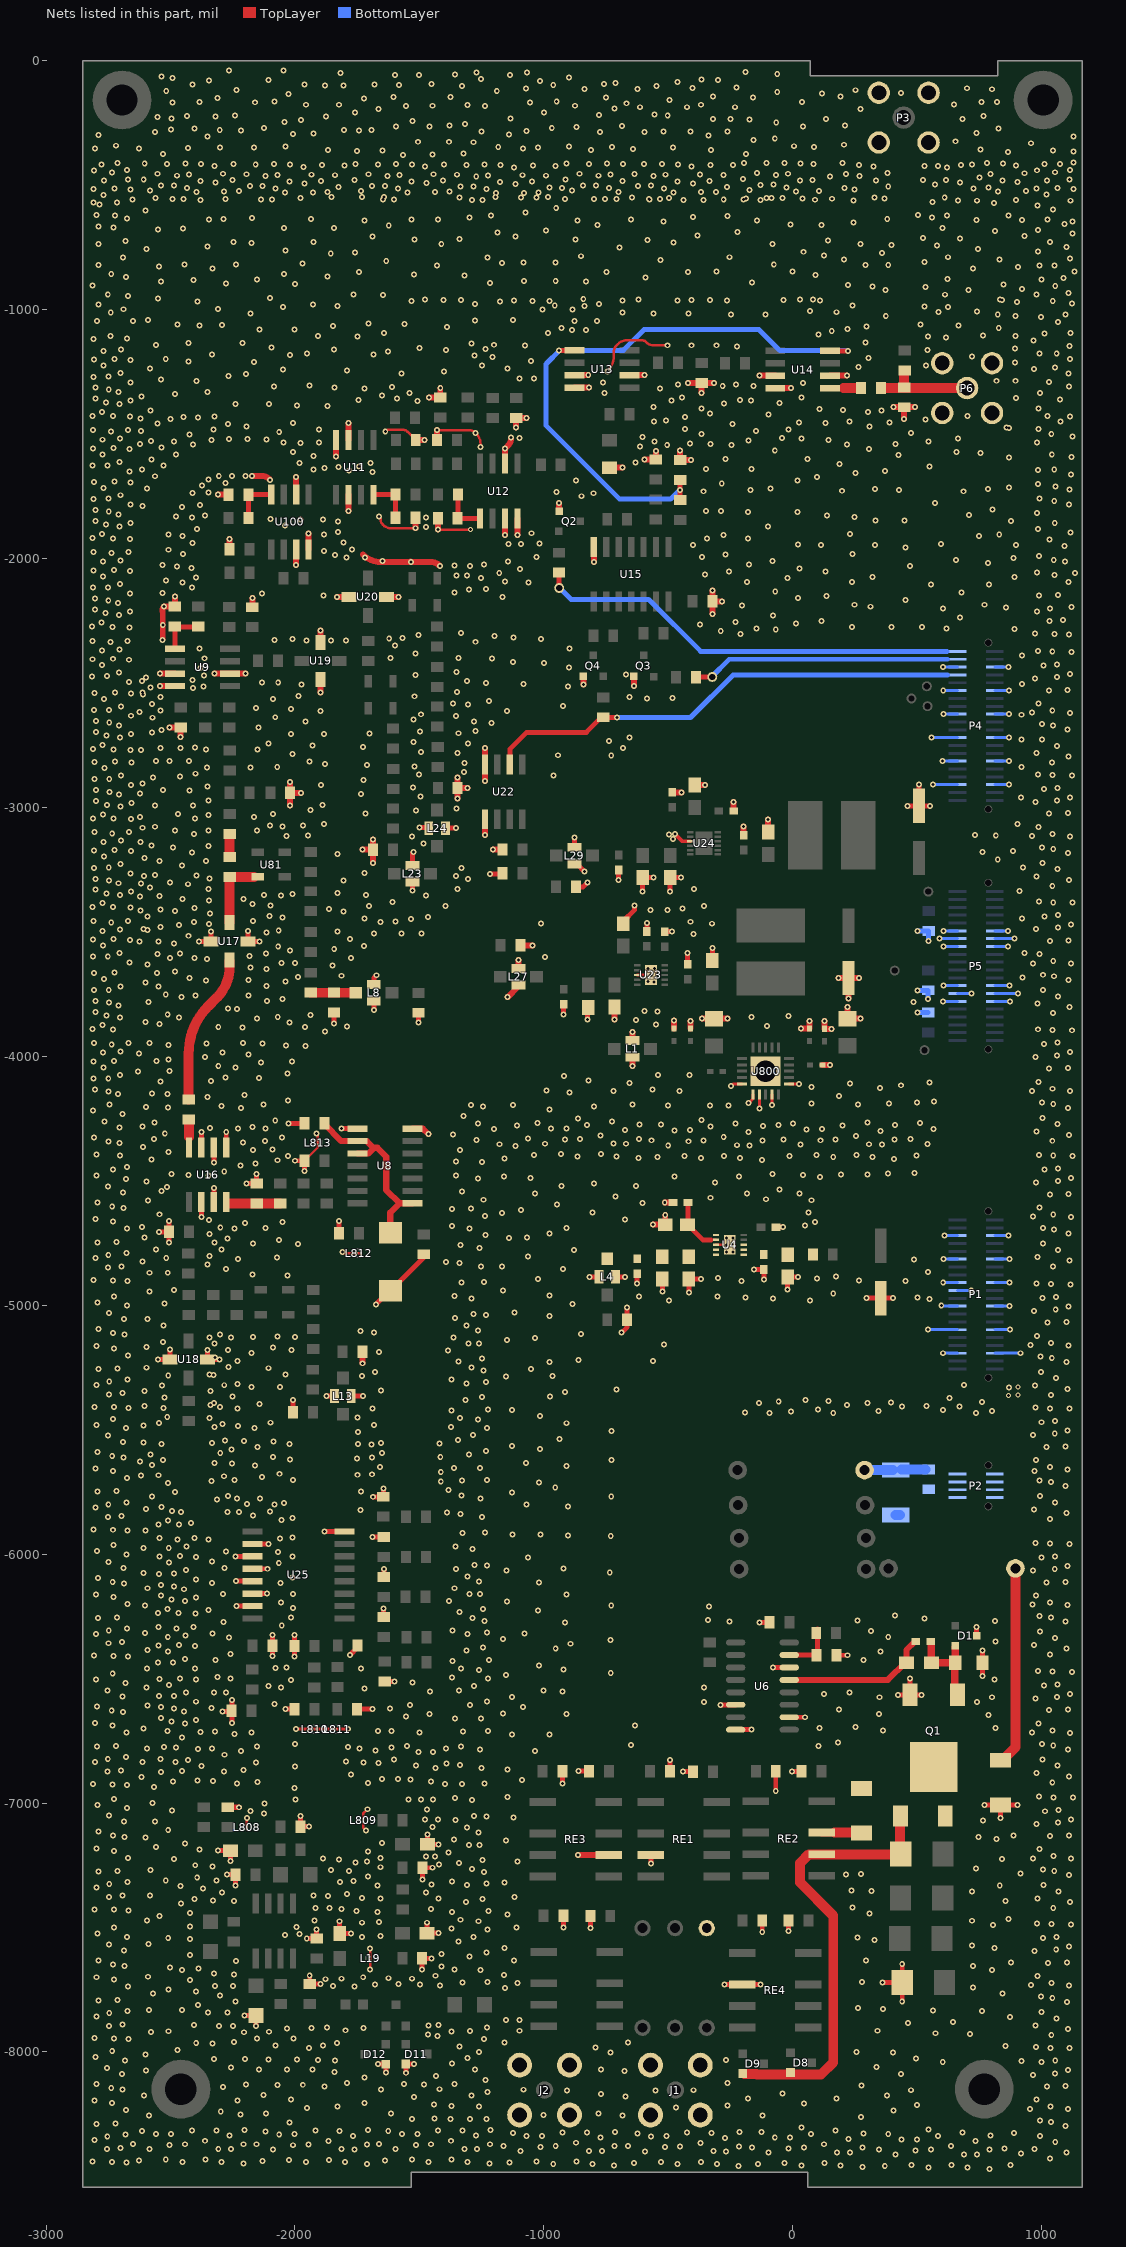
[diagram p0: the nets of this part, all layers, seen from the top]
# Altium PCB MISC109560.PcbDoc (part 5 of 7)
Units mil, origin at the board's own origin, x right, y up, seen from the top; angles counter-clockwise.
Board outline 4015.75 x 8543.31 mil, 4 copper layers (TopLayer, GND, SIG3, BottomLayer); 280 components, 173 nets, 936 pads, 3695 vias.

## Via types
v1: diameter 24, hole 12, TopLayer to BottomLayer, 3659 vias
v2: diameter 20, hole 12, TopLayer to BottomLayer, 32 vias
v3: diameter 40, hole 20, TopLayer to BottomLayer, 4 vias

## Nets (pads, with @x,y where several pads share a name; then routed paths per layer and width w, separated by ;. In a path a pad name is that pad's centre, name@x,y a point inside that pad or via, vN(x,y) a via of type N, cw(c..) or ccw(c..) an arc to the next point about the centre after c; other vN are vias at no path point) (continued)
GND: (continued)
  other v1: -2402,-3044.31 -2811,-3043.31 -2164,-3038.31 -2622,-3037.31 -2348,-3029.31 -2772,-3027.31 -2469,-3026.31 -2088,-3026.31 -1717,-3024.31 1030,-3025 1106,-3023 -1514,-3011.31 -1938,-3009.31 -1351,-3003.61 -2701,-2996.31 -2562,-2992.31 -2409,-2992.31 -1890,-2990.31 -2756,-2989.31 -2657,-2982.31 975,-2978 -2799,-2974.31 -2348,-2972.31 1063,-2972 918,-2960.31 1115,-2959 -1496,-2956.31 -2706,-2948.31 -1735,-2945.31 -2622,-2944.31 -2745,-2937.31 -2424,-2932.31 -2799,-2930.31 -2530,-2929.31 1009,-2926 -1526,-2920.31 1064,-2921 -2351,-2916.31 -1895,-2910.31 -2658,-2909.31 -2613,-2903.31 -1724,-2890.31 -2806,-2886.31 -2746,-2885.31 -2570,-2880.31 -2462,-2875.31 -2698,-2871.31 -961,-2872 1122,-2871 1044,-2870 -1501,-2868.31 986,-2867 -2399,-2864.31 -1321,-2856.61 -2766,-2841.31 -2353,-2839.31 -2179,-2838.31 -2071,-2836.31 919,-2836.31 -1520,-2834.31 -1710,-2829.31 -1879,-2824.31 -1318,-2821 -2657,-2819.31 1042,-2819 -2805,-2817.31 -2722,-2815.31 -1941,-2814.31 -2559,-2812.31 -2504,-2812.31 -2425,-2812.31 1109,-2795 -729,-2791.31 -942,-2790 -2010,-2785.31 -1347,-2780.61 979,-2781 -1493,-2777.31 -2660,-2768.31 -2618,-2768.31 -2357,-2767.31 -2150,-2767.31 -2729,-2766.31 -2812,-2765.31 -681,-2761.31 -2541,-2760.31 -2459,-2760.31 -2402,-2758.31 -1726,-2757.31 1063,-2752 -1929,-2750.31 -2773,-2749.31 -1305,-2743.61 -2107,-2742.31 -1523,-2737.31 -738,-2733.31 919,-2726.31 1002,-2727 -656,-2719.31 -2702,-2718.31 -2757,-2711.31 -2658,-2704.31 -2015,-2704.31 -1883,-2704.31 -1700,-2703.31 -1342,-2701.61 -2575,-2699.31 -2800,-2696.31 -1498,-2695.31 -1274,-2693 -2536,-2689.31 1105,-2687 -2146,-2678.31 -2707,-2670.31 1046,-2671 1001,-2665 -1211,-2661.31 -2746,-2659.31 -1957,-2654.31 -1281,-2654 -2800,-2652.31 -1524,-2647.31 -2572,-2639.31 -2079,-2637.31 -1353,-2633 -2659,-2631.31 919,-2627.31 -1493,-2625.31 1114,-2620 961,-2619 -2624,-2616.31 -1148,-2612.31 -1897,-2611.31 -2541,-2609.31 1043,-2610 -2807,-2608.31 -2747,-2607.31 -2015,-2604.31 -2157,-2600.31 -2699,-2593.31 -923,-2591.31 -1305,-2586.61 -2575,-2583.31 -1365,-2581.61 987,-2582 -1221,-2572.31 -2089,-2564.31 -2767,-2563.31 -585,-2561.31 -483,-2559.31 -2541,-2556.31 -656,-2556.31 -1986,-2552.31 -1519,-2553 -2610,-2546.31 -2658,-2541.31 -2806,-2539.31 -2613,-2538.31 -2723,-2537.31 -1348,-2535.61 1029,-2529 1105,-2527 -2409,-2520.31 -2580,-2517.31 -2368,-2514.31 -903,-2513.31 -1974,-2506.31 922,-2504.31 -1081,-2504 -1233,-2500 -2133,-2497.31 -2067,-2497.31 -2667,-2496.31 -2614,-2491.31 -1308,-2491.61 -2411,-2488.31 974,-2482 -2599,-2477.31 1062,-2476 -2815,-2473.31 -2755,-2472.31 -2366,-2470.31 -1515,-2467 -670,-2465.31 1114,-2463 -2707,-2458.31 -1350,-2455.61 -2379,-2440.31 -899,-2437.31 1008,-2430 -2775,-2428.31 1063,-2425 -1000,-2419 -1123,-2415 -2666,-2406.31 -2814,-2404.31 -2731,-2402.31 -2363,-2400.31 -1208,-2401 -1616,-2399.31 -1342,-2399.61 922,-2389.31 -1515,-2382 1121,-2375 1043,-2374 985,-2371 -2776,-2369.31 -2705,-2364.31 -2384,-2360.31 -897,-2360.31 -1598,-2349.31 -2741,-2335.31 -1274,-2334 -2813,-2330.31 -2673,-2330.31 -1954,-2329.31 -1855,-2329.31 -1794,-2329.31 -2082,-2327.31 -2533,-2326.31 -2009,-2322.31 -1012,-2323 -1621,-2321.31 -1567,-2318 -1122,-2317 -1198,-2311 -1504,-2307 1110,-2305 -210,-2303.31 1052,-2302 974,-2301 -1333,-2299 -289,-2290.31 -68,-2285.31 892,-2283.31 -146,-2280.31 618,-2280.31 -2664,-2276.31 238,-2275.31 398,-2275.31 520,-2275.31 -2733,-2274.31 -2816,-2273.31 -2531,-2266.31 -372,-2264.31 13,-2261.31 -2777,-2257.31 -230,-2254.31 116,-2250.31 1032,-2251 1087,-2246 672,-2237.31 -79,-2229.31 -2706,-2226.31 -2761,-2219.31 -2662,-2212.31 981,-2213 -2804,-2204.31 604,-2201.31 1033,-2200 857,-2196.31 312,-2193.31 1121,-2194 -203,-2188.31 249,-2185.31 770,-2185.31 -2711,-2178.31 -2750,-2167.31 453,-2166.31 -2804,-2160.31 21,-2157.31 -1165,-2154 135,-2150.31 990,-2149 -1885,-2147.31 1066,-2147 -2132,-2140.31 -2663,-2139.31 -2533,-2138.31 678,-2136.31 -1358,-2135.31 -70,-2131.31 -1301,-2124.31 -1232,-2122.31 -2811,-2116.31 -2751,-2115.31 -2414,-2115.31 556,-2104.31 789,-2104.31 -2703,-2101.31 -1062,-2096.31 -2451,-2095.31 -184,-2093.31 238,-2093.31 1108,-2094 -1156,-2092 -2518,-2087.31 -21,-2078.31 -1252,-2077.31 -2397,-2076.31 320,-2074.31 892,-2074.31 -2771,-2071.31 -1350,-2068.31 -1309,-2067.31 1052,-2066 -352,-2063.31 -1179,-2058 1134,-2057 981,-2056 -255,-2052.31 132,-2052.31 -2662,-2049.31 -2810,-2047.31 -2727,-2045.31 -1095,-2042 27,-2040.31 -2415,-2038.31 -2474,-2031.31 472,-2030.31 -1418,-2029.31 -1296,-2029.31 -1358,-2028.31 -2533,-2025.31 -175,-2024.31 -1241,-2023.31 784,-2017.31 -2772,-2012.31 -1649,-2010.31 -1143,-2011 1094,-2011 -82,-2009.31 -2701,-2007.31 656,-2006.31 1049,-2005 887,-1998.31 -1792,-1996.31 -1718,-1995.31 -1029,-1993.31 -364,-1993.31 990,-1989 -1838,-1985.31 -270,-1983.31 241,-1982.31 -2450,-1981.31 -2737,-1978.31 -2809,-1973.31 -2669,-1973.31 -1884,-1969.31 -2507,-1964.31 -1770,-1963.31 453,-1955.31 1093,-1949 -401,-1944.31 114,-1944.31 331,-1944.31 897,-1944.31 21,-1942.31 -1141,-1941.31 -1092,-1941.31 596,-1941.31 -1018,-1939.31 -2411,-1937.31 -1804,-1934.31 1032,-1924 -2662,-1920.31 -2731,-1918.31 -345,-1918.31 -179,-1918.31 -2814,-1917.31 -2452,-1908.31 748,-1908.31 -278,-1904.31 830,-1903.31 -2508,-1902.31 -1883,-1902.31 -2775,-1901.31 230,-1900.31 -1050,-1898 1116,-1895 -1827,-1893.31 -2394,-1881.31 986,-1881 -1473,-1872.31 -2704,-1870.31 -99,-1870.31 -2040,-1866.31 -2759,-1863.31 -2660,-1856.31 1053,-1857 -1826,-1851.31 878,-1849.31 -2802,-1848.31 333,-1846.31 450,-1846.31 -1977,-1843.31 -1888,-1842.31 -2098,-1841.31 -2413,-1835.31 -1473,-1835.31 249,-1832.31 -1663,-1831.31 -2478,-1830.31 138,-1827.31 -2362,-1826.31 708,-1824.31 -2709,-1822.31 981,-1817 -179,-1813.31 20,-1813.31 -2748,-1811.31 -349,-1809.31 -288,-1809.31 -2802,-1804.31 803,-1803.31 -2454,-1792.31 -2612,-1788 -2381,-1784.31 -2661,-1783.31 1111,-1783 572,-1776.31 1051,-1769 -2809,-1760.31 -2749,-1759.31 992,-1759 -849,-1749.31 -2701,-1745.31 -800,-1737.31 -2411,-1736.31 -2347,-1734.31 -949,-1733 -358,-1729.31 686,-1729.31 198,-1727.31 428,-1724.31 -169,-1723.31 1113,-1722 331,-1719.31 784,-1719.31 -2595,-1719 -89,-1717.31 -2769,-1715.31 870,-1713.31 1056,-1710 -2374,-1705.31 986,-1701 -285,-1698.31 -2279,-1695.31 -2660,-1693.31 -2808,-1691.31 -2725,-1689.31 20,-1686.31 -871,-1685.31 -2100,-1684.31 -2347,-1682.31 98,-1671.31 -2563,-1669 -2306,-1668.31 -2253,-1667.31 -2199,-1667.31 1119,-1662 252,-1656.31 -1688,-1651.31 -2665,-1649.31 371,-1647.31 -1782,-1645.31 985,-1643 -1926,-1641.31 -2614,-1641 1051,-1641 -348,-1639.31 -165,-1639.31 -1881,-1636.31 -1825,-1631.31 -1742,-1629.31 550,-1629.31 -2813,-1626.31 -2753,-1625.31 -2528,-1625 188,-1620.31 -1697,-1616.31 -1981,-1615.31 -632,-1614.31 -2705,-1611.31 -2576,-1601 -269,-1599.31 59,-1599.31 870,-1594.31 1121,-1591 -1926,-1587.31 425,-1583.31 -2773,-1581.31 -2477,-1581.31 1041,-1582 754,-1575.31 -2007,-1572.31 659,-1572.31 -72,-1565.31 -2664,-1559.31 306,-1559.31 -2812,-1557.31 -2729,-1555.31 -2536,-1554.31 -1255,-1552.31 -614,-1550.31 -504,-1542.68 -246,-1542.68 -2410,-1541.31 219,-1541.68 -330,-1539.31 -2622,-1539 -412,-1538.31 414,-1538.68 -1978,-1536.31 -2046,-1534.31 -1903,-1534.31 981,-1534 -2486,-1529.31 545,-1529.31 -555,-1528.68 -2578,-1528 -177,-1525.31 -2336,-1523.31 144,-1523.68 -2774,-1522.31 -2114,-1521.31 -2264,-1519.31 -2191,-1519.31 -2703,-1517.31 36,-1517.68 664,-1516.68 -1098,-1515.31 -42,-1514.68 -1131,-1513.31 -604,-1510.68 1124,-1510 -2424,-1501.31 -366,-1498.68 1039,-1499 -1275,-1495.31 476,-1494.68 -2063,-1491.31 -2739,-1488.31 -1637,-1488.31 -2618,-1487.31 -147,-1486.68 -2811,-1483.31 -2671,-1483.31 -16,-1481.68 -2327,-1480.31 -1903,-1480.31 -432,-1479.68 988,-1479 870,-1474.31 859,-1472.31 309,-1469.68 -2194,-1468.31 -242,-1459.68 -2269,-1458.31 -2552,-1456.31 132,-1455.68 -2007,-1454.31 389,-1453.68 25,-1452.68 -558,-1448.68 229,-1448.68 1076,-1449 -509,-1445.68 533,-1440.68 -2499,-1439.31 -2620,-1437.31 -2389,-1432 -433,-1430.68 -2662,-1429.31 -2448,-1430 1114,-1429 -2731,-1427.31 -2323,-1428 702,-1427.68 -2814,-1426.31 1024,-1426 -97,-1421.68 -332,-1417.68 -2775,-1410.31 302,-1410.68 356,-1405.68 -2581,-1404 202,-1403.68 108,-1398.68 -366,-1397.68 988,-1397 -559,-1390.68 -1870,-1387 -1992,-1384 -2704,-1379.31 -2239,-1378 -2105,-1378 -276,-1376.68 -52,-1374.68 -2759,-1372.31 -2660,-1365.31 -1508,-1366 -486,-1364.68 -168,-1364.68 -1744,-1363.31 -211,-1361.68 1074,-1361 -2802,-1357.31 -1590,-1357 897,-1355.31 -445,-1352.68 36,-1352.68 -2616,-1349.31 -1650,-1344.31 -2482,-1339 994,-1335 -1540,-1334 -756,-1333.68 -2709,-1331.31 -2351,-1331 -2748,-1320.31 -1721,-1316.31 -533,-1316.68 -2802,-1313.31 -1841,-1313 -1609,-1311.31 1111,-1309 -2084,-1308 -281,-1305.68 -157,-1305.68 -1941,-1305 -460,-1300.68 -228,-1299.68 41,-1293.68 -2661,-1292.31 -763,-1291.68 1029,-1290 -2396,-1287 819,-1285.31 895,-1285.31 -2538,-1280 -1097,-1277 -1039,-1277 -2809,-1269.31 -2749,-1268.31 -2266,-1267 -2197,-1259 1109,-1257 -1572,-1256 -2701,-1254.31 -1401,-1248 -744,-1247.68 -1790,-1244 -2047,-1240 969,-1238 -2583,-1237 -1145,-1236 1054,-1232 265,-1230.68 -2769,-1224.31 -1248,-1224.31 535,-1223.68 894,-1211.31 -2164,-1209 -2428,-1208 -1052,-1206 -2660,-1202.31 -2808,-1200.31 -2725,-1198.31 1114,-1198 -2519,-1197 304,-1194.68 -1207,-1189.31 721,-1187.68 -1279,-1183.68 -2020,-1182 -2333,-1180 -1684,-1180 -1952,-1176 991,-1175 1061,-1175 -1626,-1167 -2770,-1165.31 541,-1161.68 -2699,-1160.31 -1392,-1161 -1843,-1159 -1234,-1157.31 893,-1156.31 -1499,-1154 -2095,-1151 -224,-1147.68 1112,-1146 -1076,-1144 -406,-1142.68 -306,-1142.68 -2559,-1141 -1201,-1140.68 -1290,-1135.68 -2427,-1133 -2210,-1133 292,-1131 968,-1123 -2810,-1118 -2674,-1115 616,-1110.68 -1748,-1108 543,-1107.68 -2741,-1106 895,-1105.31 -1907,-1105 764,-1103.68 104,-1098.68 1012,-1096 -1642,-1094 1117,-1094 -983,-1092.68 157,-1085 -886,-1081.68 -831,-1081.68 -2002,-1080 -2143,-1079 221,-1077.68 828,-1073.31 -929,-1072.68 -1389,-1069 296,-1068 -1847,-1065 -2384,-1064 666,-1063.68 -2293,-1061 -2472,-1059 514,-1059 -1559,-1057 -1705,-1056 1066,-1050 -2795,-1046 -786,-1046 -2651,-1045 -876,-1045 -1277,-1043 -1124,-1042 -2590,-1041 998,-1030 895,-1025.31 374,-1025 1096,-1020 -247,-1019 -109,-1019 824,-1018.31 -2179,-1015 -559,-1015 -418,-1015 -2740,-1011 -684,-1011 177,-1010 585,-1008.68 741,-1006.31 70,-1005.31 -1005,-998.31 -884,-998.31 -2688,-998 -2310,-997 624,-989.68 -2047,-989 530,-986 -837,-984.31 -1829,-984 -956,-983.31 241,-983 -2790,-979 -1928,-979 -778,-977.31 -1277,-976 1122,-975 902,-968.31 -2392,-967 -1176.43,-966.54 -976.43,-965.54 -1532.43,-964.54 -1045.43,-964.54 -1119.43,-963.54 -463.43,-963.54 1045,-964 -684.43,-962.54 -263.43,-962.54 109,-962.31 -1333.43,-961.54 -332.43,-961.54 -37,-961.31 -1402.43,-960.54 -406.43,-960.54 841.57,-960.54 -1476.43,-959.54 28.57,-959.54 833,-959.31 -620.43,-958.54 81.57,-958.54 -841.43,-957.54 -2551,-954 -2101,-953 -2670,-944 -1646,-941 612,-939.68 -2752,-938 -1764,-938 980,-938 1109,-933 373,-921 706,-920 922,-916 534,-908 321,-907 1055,-905 -2813,-903 223,-900 848,-898 -2000,-897 -2276,-894 -1216,-892 -163,-890 -2538,-887 -831,-887 -1080,-885 -952,-885 -2408,-881 -2153,-879 999,-879 623,-876.68 1089,-872 -592,-871 -2679,-868 -1869,-867 -1319,-863 91,-861 -1522,-859 -2738,-857 -2043,-857 -748,-849 -1742,-848 -420,-848 -307,-846 -1,-846 1133,-846 -2332,-834 724,-834 905,-828 -2546,-826 -1430,-823 992,-823 1052,-823 293,-821 -2790,-820 384,-820 -76,-819 -2443,-818 -2236,-818 -1969,-815 -1167,-813 -1081,-810 -953,-810 530,-809 -1633,-805 -532,-800 206,-799 831,-799 1114,-795 -2691,-790 -1227,-790 -253,-789 625,-789 -850,-785 126,-782 -1856,-774 359,-772 -1759,-770 44,-767 986,-766 -2038,-761 -2597,-756 745,-756 -696,-749 1100,-748 -2351,-746 580,-741 398,-739 -2790,-736 272,-736 -1412,-735 -82,-735 -2174,-731 -478,-729 -1925,-728 1033,-728 -2247,-727 -2680,-723 141,-722 -583,-720 -1520,-718 -873,-718 -1338,-715 672,-714 524,-712 -1113,-706 -1689,-705 932,-704 -383,-702 1125,-693 -1186,-690 -222,-687 813,-683 -992,-681 986,-680 -2551,-677 -2449,-674 -2043,-672 -1843,-672 602,-671 -2729,-669 -2790,-666 -1623,-661 -785,-659 116,-659 -8,-657 1092,-656 244,-650 -519,-646 1125,-645 -1721,-642 -864,-642 -144,-642 739,-640 922,-640 -2346,-638 -1532,-638 -1425,-638 -649,-638 1024,-638 -2287,-636 -1936,-636 380,-636 -2675,-633 -2173,-632 -1299,-630 559,-630 -400,-628 -262,-624 621,-622 -2723,-621 -1212,-621 868,-621 -2797,-620 503,-619 -1074,-609 -2600,-602 1046,-597 -950,-592 984,-581 -2785,-578 808,-572 -2809,-570 -2715,-569 562,-567 741,-562 1116,-562 244,-561 664,-561 -2379,-559.31 -438,-559.31 897.57,-559.54 -1289.43,-558.54 -1245.43,-558.54 -358,-558.31 -128.43,-558.54 -277,-557.31 -197.43,-557.54 90,-558 -2652,-557 -2136.43,-556.54 -2092.43,-556.54 -1645.43,-556.54 -1601.43,-556.54 -576,-556.31 -914,-555.31 -707,-555.31 -576.43,-555.54 -532.43,-555.54 -2492.43,-554.54 -2448.43,-554.54 -2278,-554.31 -797.43,-554.54 -753.43,-554.54 -187,-553.31 39,-553.31 158,-554 369,-553 -2561,-551.31 -105,-551.31 -84.43,-551.54 -40.43,-551.54 -1977,-550.31 -497,-550.31 -1338,-548.31 -1092,-548.31 -1030,-548.31 -645,-548.31 329,-549 611,-549 -1853,-547.31 -1731,-547.31 -1643,-547.31 -983,-547.31 -1194,-546.31 -2769.43,-538.54 1019.57,-537.54 -1192.43,-531.54 -1080.43,-530.54 -2039.43,-529.54 -1548.43,-529.54 -1021.43,-529.54 -1927.43,-528.54 -479.43,-528.54 -2395.43,-527.54 -1868.43,-527.54 -700.43,-527.54 -367.43,-527.54 -1437.43,-526.54 -308.43,-526.54 -1378.43,-525.54 825.57,-525.54 -2284.43,-524.54 12.57,-524.54 -2225.43,-523.54 -1734.43,-523.54 105.57,-523.54 936.57,-522.54 -2581.43,-521.54 -886.43,-521.54 -173.43,-518.54 -2660.43,-516.54 -1230.43,-515.54 248,-516 1128.57,-515.54 -2808.43,-514.54 -2077.43,-513.54 -1586.43,-513.54 980.57,-513.54 -2725.43,-512.54 -517.43,-512.54 -2433.43,-511.54 -738.43,-511.54 726,-512 1063.57,-511.54 -977.43,-509.54 -926,-510 208.12,-509.93 787.57,-509.54 -25.43,-508.54 -1824.43,-507.54 -264.43,-506.54 -1334.43,-505.54 -1282.43,-504.54 384,-505 -2181.43,-503.54 -1690.43,-503.54 -2129.43,-502.54 -1638.43,-502.54 -621.43,-502.54 -2537.43,-501.54 -842.43,-501.54 -569.43,-501.54 -2485.43,-500.54 -790.43,-500.54 -129.43,-498.54 -77.43,-497.54 571,-497 -1114.43,-495.54 -1961.43,-493.54 -401.43,-492.54 -1471.43,-491.54 -2318.43,-489.54 -1175.43,-487.54 673,-488 902.57,-487.54 -2022.43,-485.54 -1531.43,-485.54 -1047.43,-485.54 -462.43,-484.54 -2378.43,-483.54 -1894.43,-483.54 -683.43,-483.54 -334.43,-482.54 -2766.43,-481.54 -1404.43,-481.54 842.57,-481.54 29.57,-480.54 334,-481 1022.57,-480.54 -2251.43,-479.54 -1760.43,-479.54 79.57,-479.54 617,-479 -2607.43,-477.54 -912.43,-477.54 523,-478 1112.57,-477.54 -2671.43,-476.54 -199.43,-474.54 750,-468 -1271.43,-465.54 150.57,-464.23 -2118.43,-463.54 -1627.43,-463.54 -558.43,-462.54 -2474.43,-461.54 -991.43,-461.54 -779.43,-461.54 268,-462 -1223.43,-460.54 -1838.43,-459.54 -1085.43,-459.54 -2070.43,-458.54 -1579.43,-458.54 -278.43,-458.54 -66.43,-458.54 -1932.43,-457.54 -1348.43,-457.54 -510.43,-457.54 -2426.43,-456.54 -731.43,-456.54 -372.43,-456.54 -2195.43,-455.54 -1704.43,-455.54 -1442.43,-455.54 -635.43,-454.54 215.12,-454.93 794.57,-454.54 -2551.43,-453.54 -2289.43,-453.54 -856.43,-453.54 -18.43,-453.54 931.57,-451.54 -143.43,-450.54 381,-450 -2734.43,-448.54 1054.57,-447.54 -2806.43,-440.54 982.57,-439.54 -2675.43,-438.54 1113.57,-437.54 -1119.43,-427.54 621,-428 -1966.43,-425.54 -406.43,-424.54 325,-425 -1476.43,-423.54 -2323.43,-421.54 -953.43,-421.54 530,-422 583,-422 -1043.43,-420.54 -1800.43,-419.54 897.57,-419.54 -1890.43,-418.54 -1173.43,-418.54 -240.43,-418.54 -1310.43,-417.54 -330.43,-417.54 267,-418 676,-418 -2020.43,-416.54 -1529.43,-416.54 -1400.43,-416.54 -1237.43,-416.54 -2776.43,-415.54 -2157.43,-415.54 -1666.43,-415.54 -460.43,-415.54 721,-416 -2376.43,-414.54 -2247.43,-414.54 -2084.43,-414.54 -1756.43,-414.54 -1593.43,-414.54 -681.43,-414.54 -597.43,-414.54 83.57,-414.54 1012.57,-414.54 1074,-415 -2513.43,-413.54 -818.43,-413.54 -524.43,-413.54 -2603.43,-412.54 -2440.43,-412.54 -908.43,-412.54 -745.43,-412.54 844.57,-412.54 31.57,-411.54 -2712.43,-410.54 -105.43,-410.54 201.12,-410.93 780.57,-410.54 -195.43,-409.54 -32.43,-409.54 1128.57,-408.54 -1566.43,-377.54 -1446.43,-376.54 -2529.43,-374.54 -188.43,-373.54 -1323.43,-372.54 866,-366 1128,-364 -1750,-362 -1649,-360 1046,-360 -1868,-358 -810,-358 -328,-358 755,-356 -641,-355 -2804,-353 -2627,-353 -1084,-353 -2429,-351 -2301,-349 -2165,-349 -1023,-349 -480,-349 -1183,-347 -726,-347 85,-347 -2037,-345 -899,-345 6,-343 -2719,-341 206,-337 957,-331 -1282,-327 -1505,-325 -1381,-325 654,-323 -158,-318 -72,-312 -2351,-303.31 1128,-303 -338,-299.31 -2790,-298 -1139,-295.31 -2008,-293.31 -1925,-291.31 738,-290 -774,-286.31 -596,-286.31 -2563,-285 -519,-284.31 -410,-284.31 -262,-284.31 -1250,-283.31 -1069,-282.31 -2217,-279.31 -1742,-279.31 -2302,-278.31 -1692,-278.31 -1803,-277.31 -2497,-275.31 -2404,-271.31 -968,-270.31 827,-271 -2125,-269.31 -868,-265.31 -1594,-264.31 -1460,-264.31 42,-263 -686,-261.31 -1378,-260.31 211,-259 -1316,-253.31 -66,-248 -2042,-246.31 -1527,-241.31 -1975,-237.31 -174,-236.31 -320,-234.31 -249,-233.31 134,-234 683,-234 -2495,-231.31 -1134,-231.31 -2553,-226 -2320,-223.31 -1876,-223.31 -2434,-221.31 767,-222 -502,-220.31 -2241,-219.31 -778,-218.31 -555,-216.31 -1758,-207.31 -1000,-207.31 -1664,-194.31 -715,-192.31 272,-193 -613,-186.31 -425,-186.31 -232,-186.31 -1553,-181.31 -1236,-181.31 -1447,-180.31 -874,-180.31 -1307,-177.31 -1955,-176.31 -1823,-176.31 -368,-176.31 648,-176 -667,-170.31 -2492,-167.31 -1056,-167.31 -2161,-166.31 37,-166 759,-166 821,-166 -2384,-164.31 -2082,-162.31 -948,-162.31 -494,-157.31 -1723,-151.31 -2311,-149.31 -751,-147.31 -159,-146.31 -1604,-145.31 -1375,-145.31 -320,-142.31 192,-143 -2025,-132.31 118,-131 435,-129 -62,-125 -1189,-121.31 -2517,-120.31 252,-118 -2234,-116.31 -837,-113.31 -623,-113.31 800,-114 -1071,-110.31 -402,-109.31 701,-110 -226,-107.31 -1328,-101.31 -548,-101.31 -1880,-99.31 -1805,-99.31 -962,-97.31 -1582,-96.31 -2412,-95.31 -1962,-94.31 -1680,-94.31 -1452,-93.31 -759,-92.31 -711,-88.31 -462,-84.31 -1015,-80.31 -2345,-78.31 -301,-77.31 -2107,-76.31 -366,-74.31 -1252,-73.31 -2492,-69.31 -899,-67.31 -2536,-62.31 -1135,-57.31 -1598,-56 -1501,-56 -1356,-54 -62,-52 -1816,-48 -1270,-46 -1068,-46 -189,-44 -2264,-38 -2045,-38
  other v2: 868,-5362 906,-5360 906,-5329 -265,-4785 -240,-4785 -265,-4756.94 -241,-4756 -266,-4729 -240,-4729 -558,-3701 -581,-3700 -569.57,-3672.94 -581,-3646 -556,-3646
"HP FILT EN": HP1.1 P4.4 R52.2 | length 1051.4
  TopLayer w20: R52.2@-388,-2476.31 HP1.1@-314,-2476.31
  BottomLayer w20: HP1.1@-326,-2475.31 -255,-2404.31 622,-2404.31
HT: L5.1 P2.2 P2.4 P2.6 P2.8
IN2: P4.8 R56.1 U22.2 | length 1977.2
  TopLayer w20: U22.2@-1137,-2840 U22.2@-1137,-2827 ; U22.2@-1136.69,-2806 U22.2@-1136.69,-2827 -1136.69,-2765.69 -1069,-2698 -829,-2698 R56.1@-775,-2644 ; R56.1@-775,-2638.31 v1(-706,-2638.31)
  BottomLayer w20: v1@-708,-2638.31 v1(-706,-2638.31) -410.31,-2638.31 -239.31,-2467.31 622,-2467.31
"LP FILT EN": LP1.1 P4.2 R51.2 | length 1740.9
  TopLayer w20: LP1.1@-938,-2129 R51.2@-938,-2049
  BottomLayer w20: LP1.1@-935,-2119 -890,-2164 -578.31,-2164 -370,-2372.31 621,-2372.31
NetC4_1: C4.1 D1.2 L2.1 Q1.1 R6.1 | length 373.9
  TopLayer w20: D1.2@654,-6375 D1.2@654,-6369
  TopLayer w30: R6.1@556,-6361 556,-6437 C4.1@557,-6437 634,-6437 L2.1@654,-6417 ; Q1.1@652,-6565.91 L2.1@652,-6422.31 ; L2.1@653,-6417 D1.2@653,-6375
NetC4_2: C4.2 R6.2 U6.13 | length 642.4
  TopLayer w20: U6.13@-13.6,-6505.31 32,-6505.31
  TopLayer w24: U6.13@-13.6,-6505.31 382.69,-6505.31 C4.2@454,-6434 ; C4.2@457,-6437 457,-6385 R6.2@490,-6352 ; R6.2@495,-6352 R6.2@495,-6351
NetC5_2: C5.2 L5.2 R7.2 | length 214
  BottomLayer w40: R7.2@284,-5661.31 C5.2@403,-5661.31 ; C5.2@438,-5659.31 L5.2@533,-5659.31
NetC6_1: C6.1 C16.2 C17.2 Q1.3 R11.1 | length 778
  TopLayer w40: C6.1@847,-6824 896,-6775 R11.1@896,-6066.31
NetC7_2: C7.2 C11.1 C12.2 L4.1 U4.9 U4.10
NetC8_2: C8.2 C9.1 L3.2 U4.1 U4.2 U4.3 U4.6
NetC14_1: C14.1 R14.1 U4.7 | length 240.2
  TopLayer w10: -345.75,-4737.25 U4.7@-308.14,-4737.25
  TopLayer w20: C14.1@-422,-4676 -360.75,-4737.25 -328.8,-4737.25 ; C14.1@-421,-4671 R14.1@-421,-4587
NetC16_1: C16.1 D5.1 D8.2 D9.2 RE2.6 | length 1781
  TopLayer w30: D9.2@-201,-8086.59 D9.2@-193,-8086.59 ; D5.1@431.54,-7231 D5.1@438.22,-7237.69
  TopLayer w40: D9.2@-193,-8089.59 -144.77,-8089.59 ; -143.58,-8090.78 114.22,-8090.78 163,-8042 163,-7452.59 29,-7318.59 29,-7241.59 64.59,-7206 D5.1@413,-7206 ; C16.1@432,-7072 432,-7200 434,-7202 D5.1@434,-7205
NetC17_1: C17.1 RE2.7 | length 155.3
  TopLayer w30: RE2.7@116.69,-7118.98 174.39,-7118.98
  TopLayer w40: RE2.7@168,-7118.59 184,-7118.59 ; 174.39,-7118.98 C17.1@255.98,-7118.98
NetC18_1: C18.1 R16.1 U6.15 | length 180
  TopLayer w20: U6.15@14,-6405.31 C18.1@95,-6405.31 ; C18.1@99,-6400.31 R16.1@99,-6301.31
NetC41_1: C41.1 U14.1 | length 64
  TopLayer w40: 204,-1314.68 C41.1@268,-1314.68
NetC41_2: C41.2 P6.5 R1.1 R32.1 | length 394.7
  TopLayer w40: C41.2@363,-1314.68 P6.5@701,-1314.68 ; R32.1@448,-1311.68 R1.1@448,-1255
NetC42_1: C42.1 R27.1 U9.5 | length 176.5
  TopLayer w20: U9.5@-2481.59,-2362.27 -2481.59,-2274.9 -2394.41,-2274.9 R27.1@-2393,-2276.31
NetC43_2: C43.2 R28.2 U100.4 | length 175.2
  TopLayer w20: R28.2@-2185.96,-1835.35 C43.2@-2185.96,-1742.72 U100.4@-2103.41,-1742.72
NetC44_1: C44.1 R29.1 U11.4 | length 170.8
  TopLayer w20: U11.4@-1674.59,-1742.72 -1596.41,-1742.72 C44.1@-1596.41,-1835.35
NetC45_1: C45.1 R30.1 U12.5 | length 176.2
  TopLayer w20: R30.1@-1345.41,-1742.35 -1345.41,-1832.9 -1340,-1838.31 U12.5@-1262,-1838.31
NetC46_1: C46.1 R31.1 U13.5 U14.4 | length 2494.7
  TopLayer w20: v1@-938,-1163.09 U13.5@-875.96,-1163.09 ; v1(-453,-1723.31) v1@-452,-1723.31 ; R31.1@-452,-1765.31 v1@-452,-1723.31 ; C46.1@-452,-1691.31 v1@-452,-1723.31 ; U14.4@150.04,-1165.09 v1(221.59,-1165.09)
  BottomLayer w20: -992,-1217.68 -992,-1464.68 -695.37,-1761.31 -608,-1761.31 ; -989,-1215.68 -936.41,-1163.09 -680.41,-1163.09 -597,-1079.68 -136,-1079.68 -51,-1164.68 v1@220,-1164.68 ; -669,-1761.31 -608,-1761.31 ; v1(-453,-1723.31) -491,-1761.31 -608,-1761.31
  other v1: -938,-1163.68
NetC47_2: C47.2 R35.1 U16.4 | length 204.8
  TopLayer w40: U16.4@-2263.74,-4590.31 R35.1@-2058.96,-4590.31
NetC48_2: C48.2 L8.3 R36.1 | length 170
  TopLayer w40: R36.1@-1937.04,-3744.27 L8.3@-1767,-3744.27
NetC49_1: C49.1 C50.1 U8.1 U8.9 U8.10 | length 754.4
  TopLayer w25: C50.1@-1882.96,-4263.31 -1882.96,-4271.31 -1813.92,-4340.35 U8.9@-1748.37,-4340.35 -1710.92,-4340.35 -1686.96,-4364.31 ; U8.10@-1748.37,-4390.35 -1705,-4390.35 -1685.96,-4371.31 ; -1685.96,-4367.31 -1668.69,-4367.31 -1633,-4403 -1633,-4537 -1579.65,-4590.35 ; C49.1@-1617,-4688 -1617,-4627.69 -1579.65,-4590.35 ; U8.1@-1528.37,-4590.35 -1579.65,-4590.35
NetC51_1: C51.1 U17.1 | length 606.4
  TopLayer w40: C51.1@-2426.96,-4173.31 -2426.96,-3988.37 cw(c-2157.99,-3988.37) -2348.18,-3798.18 -2312.65,-3762.65 ccw(c-2432.51,-3642.79) -2263,-3642.79 U17.1@-2263,-3616
NetC51_2: C51.2 U16.8 | length 62
  TopLayer w40: -2426,-4324 C51.2@-2426,-4262
NetC52_1: C52.1 L10.2 | length 69.4
  TopLayer w40: C52.1@-2262.96,-3187.72 L10.2@-2262.96,-3118.35
NetC52_2: C52.2 U17.3 U81.1 | length 276.7
  TopLayer w40: U17.3@-2262.96,-3462.72 C52.2@-2262.96,-3283 ; C52.2@-2262,-3279 U81.1@-2165,-3279